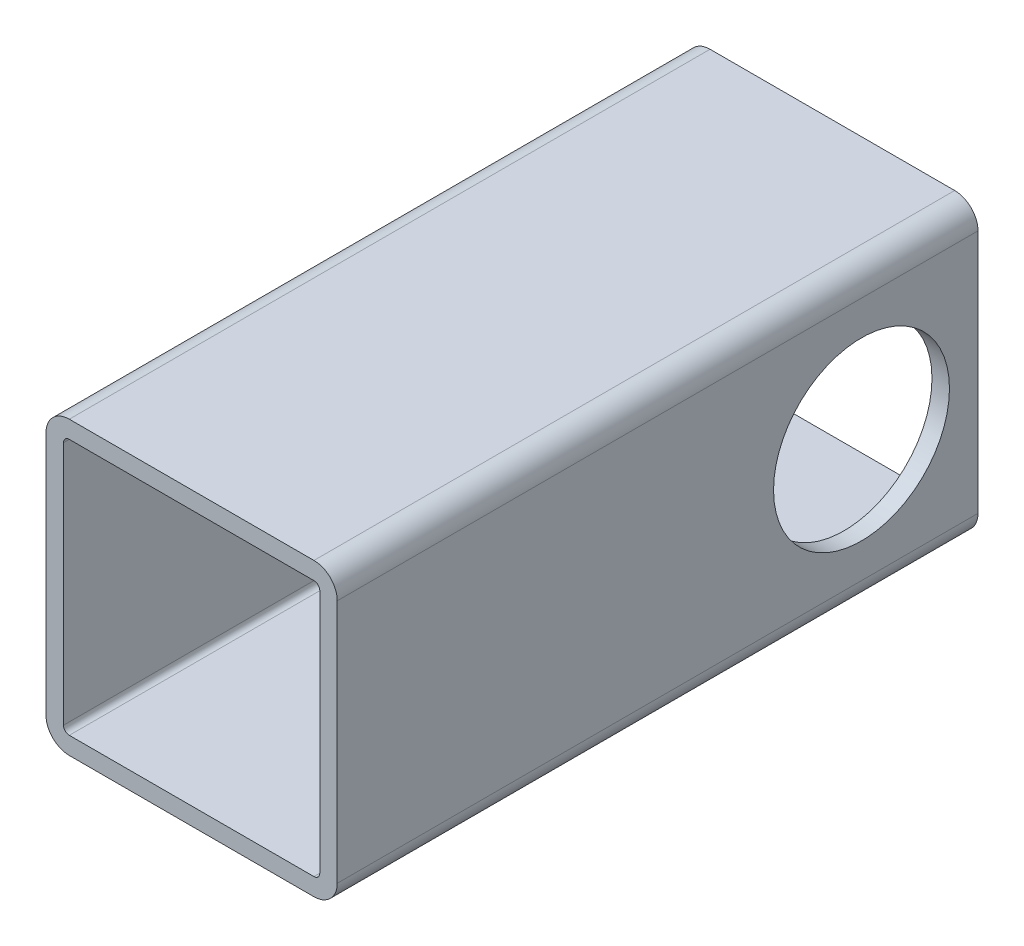
from build123d import *

# Parameters (mm, degrees)
EXTRUDE_THIN1_DEPTH = 110
SKETCH2_R           = 15.1
CUT_EXTRUDE1_DEPTH  = 124.389626793


with BuildPart() as part:
    # Sketch1 → Extrude-Thin1 (new body)
    with BuildSketch(Plane.XY):
        with BuildLine():
            Line((-25, 21), (-25, -21))
            ThreePointArc((-25, -21), (-23.828427125, -23.828427125), (-21, -25))
            Line((-21, -25), (21, -25))
            ThreePointArc((21, -25), (23.828427125, -23.828427125), (25, -21))
            Line((25, -21), (25, 21))
            ThreePointArc((25, 21), (23.828427125, 23.828427125), (21, 25))
            Line((21, 25), (-21, 25))
            ThreePointArc((-21, 25), (-23.828427125, 23.828427125), (-25, 21))
        make_face()
        with BuildLine():
            Line((-22, 21), (-22, -21))
            ThreePointArc((-22, -21), (-21.707106781, -21.707106781), (-21, -22))
            Line((-21, -22), (21, -22))
            ThreePointArc((21, -22), (21.707106781, -21.707106781), (22, -21))
            Line((22, -21), (22, 21))
            ThreePointArc((22, 21), (21.707106781, 21.707106781), (21, 22))
            Line((21, 22), (-21, 22))
            ThreePointArc((-21, 22), (-21.707106781, 21.707106781), (-22, 21))
        make_face(mode=Mode.SUBTRACT)
    extrude(amount=EXTRUDE_THIN1_DEPTH)

    # Sketch2 → Cut-Extrude1 (cut, through all)
    with BuildSketch(Plane(origin=(25, 0, 0), x_dir=(0, 0, -1), z_dir=(1, 0, 0))):
        with Locations((-20, 0)):
            Circle(SKETCH2_R)
    extrude(amount=-CUT_EXTRUDE1_DEPTH, mode=Mode.SUBTRACT)


solid = part.part
